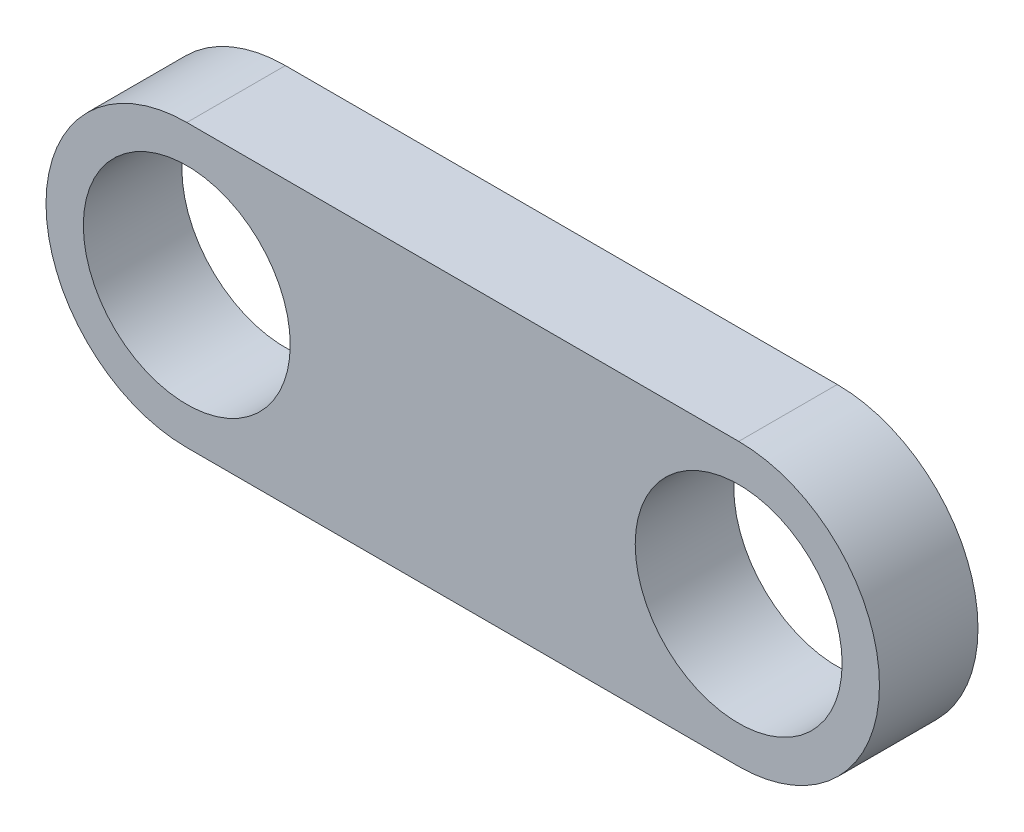
SolidWorks part; units mm, degrees
ref_plane "Front Plane" through (0, 0, 0) normal (0, 0, 1) x (1, 0, 0)
ref_plane "Top Plane" through (0, 0, 0) normal (0, 1, 0) x (1, 0, 0)
ref_plane "Right Plane" through (0, 0, 0) normal (1, 0, 0) x (0, 0, -1)
other "Configuration Table"
sketch "Sketch1" plane through (0, 0, 0) normal (0, 0, 1) x (1, 0, 0)
  line L0 (7.4641, 0.0077) -> (27.0657, 0) construction
  line L1 (7.466, 5.0077) -> (27.0676, 5)
  line L2 (7.4621, -4.9923) -> (27.0637, -5)
  circle A1 centre (7.4641, 0.0077) radius 3.6746
  circle A3 centre (27.0657, 0) radius 3.6746
  arc A4 (7.466, 5.0077) -> (7.4621, -4.9923) centre (7.4641, 0.0077) ccw
  arc A5 (27.0637, -5) -> (27.0676, 5) centre (27.0657, 0) ccw
  point P3 (17.2649, 0.0039)
extrude "Boss-Extrude1" add sketch "Sketch1" along normal up to surface (3.5 mm away) contours A5 L1 A4 L2
sketch "Sketch2" plane through (0, 0, 0) normal (0, 0, -1) x (-1, 0, 0)
  circle A1 centre (-27.0657, 0) radius 3.6746
  circle A2 centre (-7.4641, 0.0077) radius 3.6746
extrude "Cut-Extrude1" cut sketch "Sketch2" against normal up to surface (3.5 mm away)
